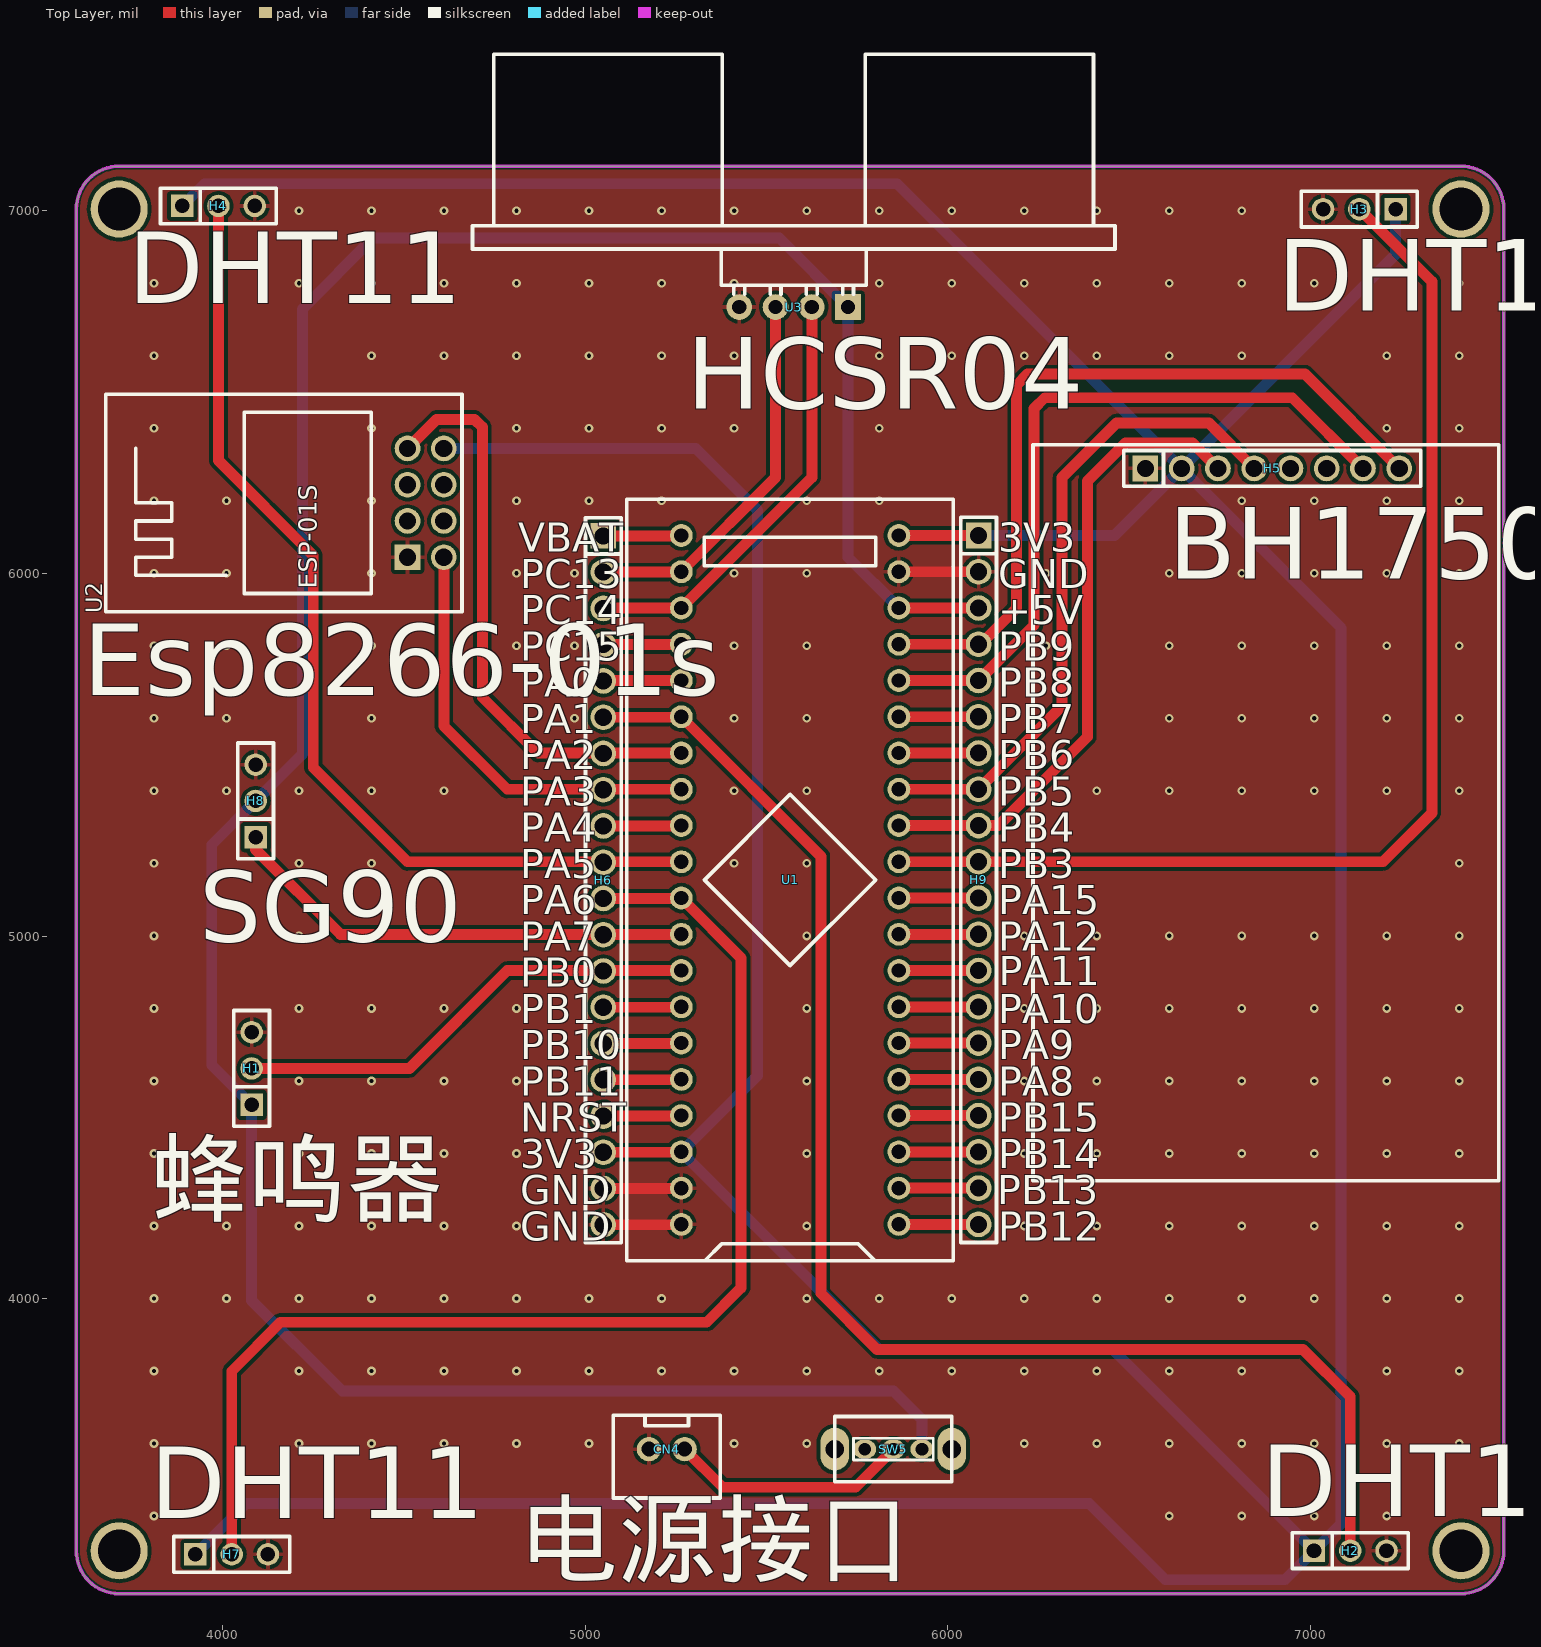
[diagram p0: Top Layer view]
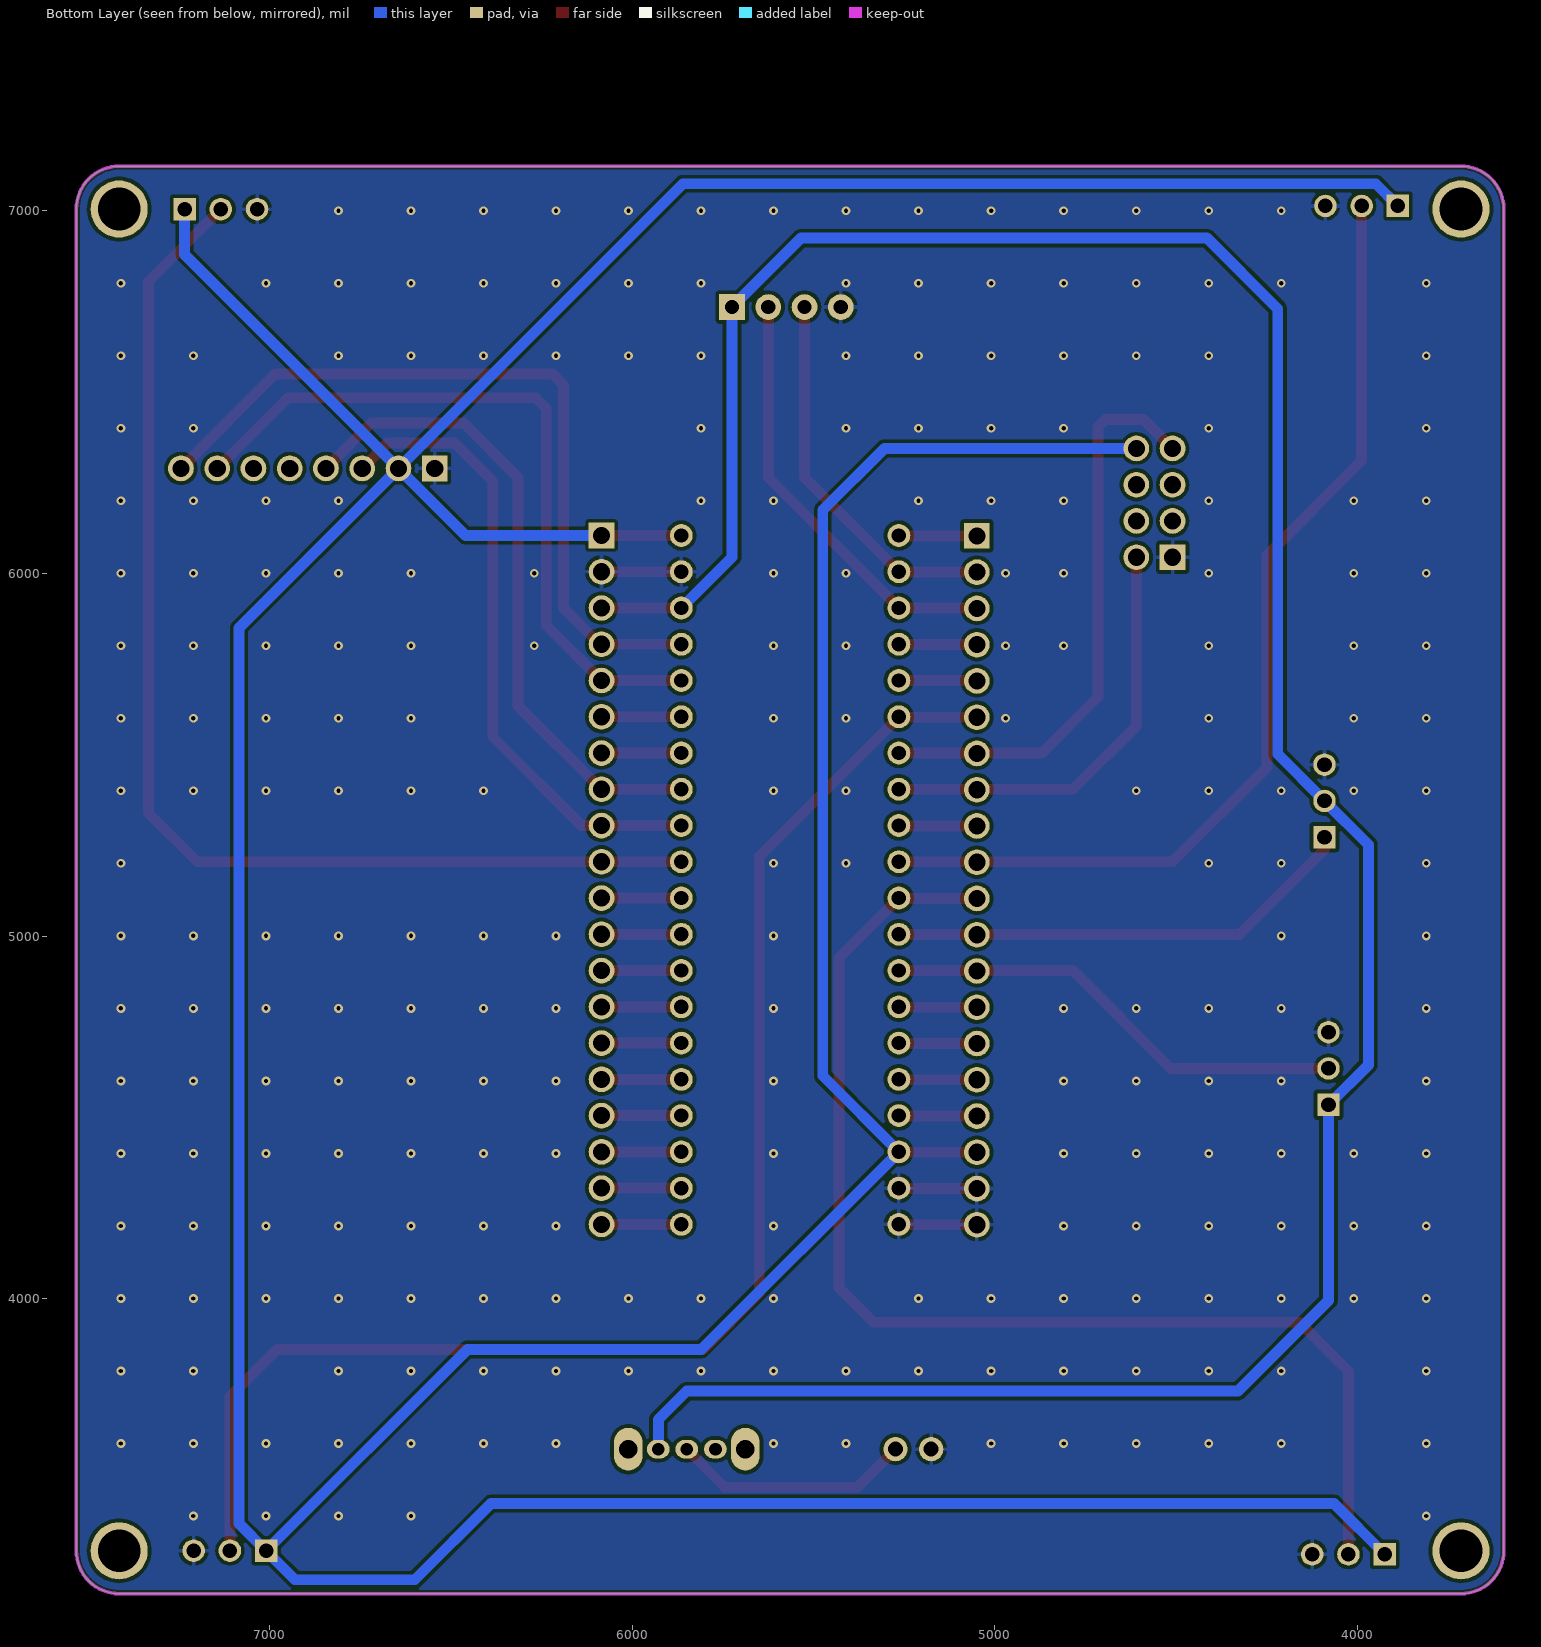
[diagram p1: Bottom Layer view, seen from below]
# Altium PCB MISC50977.pcbdoc
Units mil, origin at the board's own origin, x right, y up, seen from the top; angles counter-clockwise.
Board outline 3937.01 x 3937.01 mil, 2 copper layers (Top Layer, Bottom Layer), stack 62.206 mil thick; 14 components, 40 nets, 129 pads, 241 vias.

## Layer stack, top to bottom
Top Solder Mask Layer: solder mask 0.394, Dk 3.3
Top Layer: signal copper 1.379
Dielectric1: surface 59.449, FR4, Dk 4.5
Bottom Layer: signal copper 1.378
Bottom Solder Mask Layer: solder mask 0.394, Dk 3.3

## Board outline
3714.61,7123.5 ccw(c3714.61,7005.39) 3596.5,7005.39 3596.5,3304.61 ccw(c3714.61,3304.61) 3714.61,3186.5 7415.39,3186.5 ccw(c7415.39,3304.61) 7533.5,3304.61 7533.5,7005.39 ccw(c7415.39,7005.39) 7415.39,7123.5 3714.61,7123.5

## Design rules (kind name [scope] priority, off if disabled: settings)
BoardOutlineClearance copperThickness2oz_1 [All] p2 off: genericclearance=7.99 ignorepadtopadclearanceinfootprint=FALSE except(0: Arc-SplitContinuation Track-SplitContinuation SMDPad-SplitContinuation THPad-SplitContinuation Via-SplitContinuation Fill-SplitContinuation Region-SplitContinuation Poly-SplitContinuation Text-SplitContinuation Hole-SplitContinuation; 5.98: Arc-CutoutEdge SMDPad-CutoutEdge THPad-CutoutEdge Via-CutoutEdge Fill-CutoutEdge Region-CutoutEdge Text-CutoutEdge; 6.93: Hole-OutlineEdge Hole-CutoutEdge; 10: Poly-OutlineEdge Poly-CutoutEdge; 11.81: Arc-OutlineEdge Track-OutlineEdge SMDPad-OutlineEdge THPad-OutlineEdge Via-OutlineEdge Fill-OutlineEdge Region-OutlineEdge Text-OutlineEdge Track-CutoutEdge)
BoardOutlineClearance copperThickness1oz_1 [All] p4: genericclearance=4.02 ignorepadtopadclearanceinfootprint=FALSE except(0: Arc-SplitContinuation Track-SplitContinuation SMDPad-SplitContinuation THPad-SplitContinuation Via-SplitContinuation Fill-SplitContinuation Region-SplitContinuation Poly-SplitContinuation Text-SplitContinuation Hole-SplitContinuation; 6: SMDPad-CutoutEdge THPad-CutoutEdge Via-CutoutEdge Fill-CutoutEdge Region-CutoutEdge Text-CutoutEdge; 6.93: Hole-OutlineEdge Hole-CutoutEdge; 10: Poly-OutlineEdge Poly-CutoutEdge; 11.8: Arc-OutlineEdge Track-OutlineEdge SMDPad-OutlineEdge THPad-OutlineEdge Via-OutlineEdge Fill-OutlineEdge Region-OutlineEdge Text-OutlineEdge; 11.81: Arc-CutoutEdge Track-CutoutEdge)
Clearance copperThickness2oz [All] p1 off: gap=7.99 ignorepadtopadclearanceinfootprint=FALSE except(5.98: SMDPad-Track SMDPad-SMDPad THPad-Track SMDPad-THPad THPad-THPad Track-Via SMDPad-Via THPad-Via Via-Via Fill-Track Region-Track Fill-SMDPad Region-SMDPad Fill-THPad Region-THPad Fill-Via Region-Via Fill-Fill Fill-Region Region-Region Arc-Track Arc-SMDPad Arc-THPad Arc-Via Fill-Arc Region-Arc Arc-Arc Text-Track SMDPad-Text Text-THPad Text-Via Fill-Text Region-Text Arc-Text Text-Text; 6.93: Hole-Track Hole-SMDPad Hole-THPad Hole-Via Fill-Hole Region-Hole Hole-Arc Hole-Text; 10: Poly-Track Poly-SMDPad Poly-THPad Poly-Via Poly-Fill Poly-Region Poly-Poly Poly-Arc Poly-Text Poly-Hole)
Clearance copperThickness1oz [All] p3: gap=4.02 ignorepadtopadclearanceinfootprint=FALSE except(5.98: SMDPad-Track SMDPad-SMDPad THPad-Track SMDPad-THPad THPad-THPad Track-Via SMDPad-Via THPad-Via Via-Via Fill-Track Region-Track Fill-SMDPad Region-SMDPad Fill-THPad Region-THPad Fill-Via Region-Via Fill-Fill Fill-Region Region-Region; 6: Arc-Track Arc-SMDPad Arc-THPad Arc-Via Fill-Arc Region-Arc Arc-Arc Text-Track SMDPad-Text Text-THPad Text-Via Fill-Text Region-Text Arc-Text Text-Text; 6.93: Hole-Track Hole-SMDPad Hole-THPad Hole-Via Fill-Hole Region-Hole Hole-Arc Hole-Text; 10: Poly-Track Poly-SMDPad Poly-THPad Poly-Via Poly-Fill Poly-Region Poly-Poly Poly-Arc Poly-Text Poly-Hole)
DiffPairsRouting differentialPair [All] p1: maxlimit=6 minlimit=6 mostfreqgap=6 toplayer_minwidth=5 toplayer_prefwidth=10 toplayer_maxwidth=100 toplayer_mingap=6 toplayer_prefgap=6 toplayer_maxgap=6 bottomlayer_minwidth=5 bottomlayer_prefwidth=10 bottomlayer_maxwidth=100 bottomlayer_mingap=6 bottomlayer_prefgap=6 bottomlayer_maxgap=6 maxuncoupledlength=10
HoleToHoleClearance otherClearance [All] p1: gap=11.81 allowstackedmicrovias=TRUE
Length netLength [All] p1: minlimit=0 maxlimit=0
MatchedLengths netLengthTolerance [All] p1: tolerance=1000
PasteMaskExpansion pasteMaskExpansion [All] p1: expansion=0
PlaneConnect innerPlane [All] p1: planeconnectstyle=Relief reliefexpansion=20 reliefentries=4 reliefconductorwidth=10 reliefairgap=10
PolygonConnect copperRegion [All] p1: connectstyle=Relief reliefconductorwidth=10 reliefentries=4 polygonreliefangle="90 Angle" airgapwidth=10 via.connectstyle=Relief via.reliefconductorwidth=10 via.reliefentries=4 via.polygonreliefangle="90 Angle" via.airgapwidth=10
RoutingVias viaSize [All] p1: holewidth=12.01 width=24.02 viastyle="Through Hole" minholewidth=11.81 minwidth=19.68 maxholewidth=248.03 maxwidth=393.7
SolderMaskExpansion solderMaskExpansion [IsVia] p1: expansion=-1000 istentingtop=TRUE
SolderMaskExpansion solderMaskExpansion [All] p2: expansion=2 istentingtop=FALSE
Width copperThickness2oz_2 [All] p1 off: maxlimit=100 minlimit=8 preferedwidth=10
Width copperThickness1oz_2 [All] p2: maxlimit=100 minlimit=5 preferedwidth=10

## Components (designator, comment, footprint, x,y, rotation, side; value= is the part's Value field where it differs from the comment)
CN4 "XH2.54*2P_直插" CONN-TH_2P-P2.50-XH2.54-2P 5225,3585 r0 top
H1 "" HDR-TH_3P-P2.54-V-F 4080,4635 r90 top
H2 "" HDR-TH_3P-P2.54-V-F 7110,3305 r0 top
H3 "" HDR-TH_3P-P2.54-V-F 7135,7005 r180 top
H4 "" HDR-TH_3P-P2.54-V-F 3988.48,7013.84 r0 top
H5 "" HDR-TH_8P-P2.54-V-F-1 6895,6290 r0 top
H6 "" HDR-TH_20P-P2.54-V-M-1 5049.9,5153.84 r270 top
H7 "" HDR-TH_3P-P2.54-V-F 4025,3295 r0 top
H8 "" HDR-TH_3P-P2.54-V-F 4091.04,5372.91 r90 top
H9 "" HDR-TH_20P-P2.54-V-M-1 6085,5155 r270 top
SW5 "" 拨动开关 5855,3585 r180 top
U1 "STM32F103C8T6-Card" CONN-TH_L53.3-W22.9_STM32F103C8T6-CARD 5565,5155 r90 top
U2 "ESP-01S" WIFIM-TH_ESP-01S 4560,6195 r90 top
U3 "HC-SR04" TH_HC-SR04V 5575,6735 r180 top

## Footprints (in the part's own frame and the unit in brackets; to place one, negate y for a bottom-side part, rotate by r counter-clockwise, add the part's x,y. Pads: shape width x height; smd on the part's side, far side on the other; paste and mask are expansions set on the pad)
CONN-TH_2P-P2.50-XH2.54-2P [mm]
  round 1.7 hole 1.05 paste+0 mask+0.05: 1(1.25,0) 2(-1.25,0)
  silkscreen extent -3.75,-3.42 3.75,2.37
CONN-TH_L53.3-W22.9_STM32F103C8T6-CARD [mm]
  round 1.6 hole 1: 1(-24.13,-7.62) 2(-21.59,-7.62) 3(-19.05,-7.62) 4(-16.51,-7.62) 5(-13.97,-7.62) 6(-11.43,-7.62) 7(-8.89,-7.62) 8(-6.35,-7.62) 9(-3.81,-7.62) 10(-1.27,-7.62) 11(1.27,-7.62) 12(3.81,-7.62) 13(6.35,-7.62) 14(8.89,-7.62) 15(11.43,-7.62) 16(13.97,-7.62) 17(16.51,-7.62) 18(19.05,-7.62) 19(21.59,-7.62) 20(24.13,-7.62) 21(24.13,7.62) 22(21.59,7.62) 23(19.05,7.62) 24(16.51,7.62) 25(13.97,7.62) 26(11.43,7.62) 27(8.89,7.62) 28(6.35,7.62) 29(3.81,7.62) 30(1.27,7.62) 31(-1.27,7.62) 32(-3.81,7.62) 33(-6.35,7.62) 34(-8.89,7.62) 35(-11.43,7.62) 36(-13.97,7.62) 37(-16.51,7.62) 38(-19.05,7.62) 39(-21.59,7.62) 40(-24.13,7.62)
  silkscreen extent -26.67,-11.43 26.67,11.43
HDR-TH_3P-P2.54-V-F [mil]
  rect 62x62 hole 40.16: 1(-100,0)
  round 62 hole 40.16: 2(0,0) 3(100,0)
  silkscreen extent -160,-49 160,49
HDR-TH_8P-P2.54-V-F-1 [mm]
  rect 1.8x1.8 hole 1.2: 1(-8.89,0)
  round 1.8 hole 1.2: 2(-6.35,0) 3(-3.81,0) 4(-1.27,0) 5(1.27,0) 6(3.81,0) 7(6.35,0) 8(8.89,0)
  silkscreen extent -10.41,-1.25 10.41,1.25
HDR-TH_20P-P2.54-V-M-1 [mm]
  rect 1.8x1.8 hole 1.2: 1(-24.13,0)
  round 1.8 hole 1.2: 2(-21.59,0) 3(-19.05,0) 4(-16.51,0) 5(-13.97,0) 6(-11.43,0) 7(-8.89,0) 8(-6.35,0) 9(-3.81,0) 10(-1.27,0) 11(1.27,0) 12(3.81,0) 13(6.35,0) 14(8.89,0) 15(11.43,0) 16(13.97,0) 17(16.51,0) 18(19.05,0) 19(21.59,0) 20(24.13,0)
  silkscreen extent -25.4,-1.25 25.4,1.25
TH_HC-SR04V [mm]
  rect 1.8x1.8 hole 1.001: 1(-3.81,0)
  round 1.8 hole 1.001: 2(-1.27,0) 3(1.27,0) 4(3.81,0)
  silkscreen extent -22.5,-17.7 22.5,-0.89
WIFIM-TH_ESP-01S [mm]
  rect 1.8x1.8 hole 1.2: 1(-3.81,1.27)
  round 1.8 hole 1.2: 2(-1.27,1.27) 3(1.27,1.27) 4(3.81,1.27) 5(3.81,-1.27) 6(1.27,-1.27) 7(-1.27,-1.27) 8(-3.81,-1.27)
  silkscreen extent -7.62,-2.54 7.62,22.4
拨动开关 [mil]
  oval 63x51.2 hole 35.4 paste+0 mask+2: 1(-73.4,0) 2(5,0) 3(84,0)
  oval 78.7x118.1 hole 51.2 paste+0 mask+2: 4(166.7,0) 5(-156.1,0)
  silkscreen extent -156,-90 167,90

## Free pads (board coordinates)
  round 157.48 hole 118.11: 1(3714.61,7005.39) 1(3714.61,3304.61) 1(7415.39,7005.39) 1(7415.39,3304.61)

## Via types
v1: diameter 24.02, hole 12, Top Layer to Bottom Layer, 241 vias

## Nets (pads, with @x,y where several pads share a name; then routed paths per layer and width w, separated by ;. In a path a pad name is that pad's centre, name@x,y a point inside that pad or via, vN(x,y) a via of type N, cw(c..) or ccw(c..) an arc to the next point about the centre after c; other vN are vias at no path point)
$1N9: CN4.1 SW5.2 | length 662.8
  Top Layer w30: CN4.1 5379.22,3480 5745,3480 SW5.2
+5V: H1.1 H8.2 H9.3 SW5.1 U1.18 U3.1 | length 7722.6
  Top Layer w30: U1.18 H9.3
  Bottom Layer w30: U1.18 5725,6045 U3.1 5535,6925 4415,6925 4220,6730 4220,5501.87 H8.2 3970,5251.87 3970,4645 H1.1 4080,3995 4330,3745 5850,3745 5928.4,3666.6 SW5.1
GND: CN4.2 H1.3 H2.3 H3.3 H4.3 H5.1 H6.19 H6.20 H7.3 H8.3 H9.2 U1.19 U1.39 U1.40 U2.1 U3.4 | length 651.2
  Top Layer w30: H6.20 5263.83,4203.84 U1.40 ; H6.19 5263.83,4303.84 U1.39 ; U1.19 H9.2
  other v1: 3810.6,3400.6 6610.6,3400.6 6810.6,3400.6 7010.6,3400.6 7210.6,3400.6 3810.6,3600.6 4210.6,3600.6 4410.6,3600.6 4610.6,3600.6 4810.6,3600.6 5010.6,3600.6 5410.6,3600.6 5610.6,3600.6 6210.6,3600.6 6410.6,3600.6 6610.6,3600.6 6810.6,3600.6 7010.6,3600.6 7210.6,3600.6 7410.6,3600.6 3810.6,3800.6 4210.6,3800.6 4410.6,3800.6 4610.6,3800.6 4810.6,3800.6 5010.6,3800.6 5210.6,3800.6 5410.6,3800.6 5610.6,3800.6 5810.6,3800.6 6010.6,3800.6 6210.6,3800.6 6410.6,3800.6 6610.6,3800.6 6810.6,3800.6 7210.6,3800.6 7410.6,3800.6 3810.6,4000.6 4010.6,4000.6 4210.6,4000.6 4410.6,4000.6 4610.6,4000.6 4810.6,4000.6 5010.6,4000.6 5210.6,4000.6 5610.6,4000.6 5810.6,4000.6 6010.6,4000.6 6210.6,4000.6 6410.6,4000.6 6610.6,4000.6 6810.6,4000.6 7010.6,4000.6 7210.6,4000.6 7410.6,4000.6 3810.6,4200.6 4010.6,4200.6 4210.6,4200.6 4410.6,4200.6 4610.6,4200.6 4810.6,4200.6 5610.6,4200.6 6210.6,4200.6 6410.6,4200.6 6610.6,4200.6 6810.6,4200.6 7010.6,4200.6 7210.6,4200.6 7410.6,4200.6 3810.6,4400.6 4010.6,4400.6 4210.6,4400.6 4410.6,4400.6 4610.6,4400.6 4810.6,4400.6 5610.6,4400.6 6210.6,4400.6 6410.6,4400.6 6610.6,4400.6 6810.6,4400.6 7010.6,4400.6 7210.6,4400.6 7410.6,4400.6 3810.6,4600.6 4210.6,4600.6 4410.6,4600.6 4610.6,4600.6 4810.6,4600.6 5610.6,4600.6 6210.6,4600.6 6410.6,4600.6 6610.6,4600.6 6810.6,4600.6 7010.6,4600.6 7210.6,4600.6 7410.6,4600.6 3810.6,4800.6 4210.6,4800.6 4410.6,4800.6 4610.6,4800.6 4810.6,4800.6 5610.6,4800.6 6210.6,4800.6 6410.6,4800.6 6610.6,4800.6 6810.6,4800.6 7010.6,4800.6 7210.6,4800.6 7410.6,4800.6 3810.6,5000.6 4210.6,5000.6 5610.6,5000.6 6210.6,5000.6 6410.6,5000.6 6610.6,5000.6 6810.6,5000.6 7010.6,5000.6 7210.6,5000.6 7410.6,5000.6 3810.6,5200.6 4210.6,5200.6 4410.6,5200.6 5410.6,5200.6 5610.6,5200.6 7410.6,5200.6 3810.6,5400.6 4010.6,5400.6 4210.6,5400.6 4410.6,5400.6 4610.6,5400.6 5410.6,5400.6 5610.6,5400.6 6410.6,5400.6 6610.6,5400.6 6810.6,5400.6 7010.6,5400.6 7210.6,5400.6 7410.6,5400.6 3810.6,5600.6 4010.6,5600.6 4410.6,5600.6 4970.6,5600.6 5410.6,5600.6 5610.6,5600.6 6610.6,5600.6 6810.6,5600.6 7010.6,5600.6 7210.6,5600.6 7410.6,5600.6 3810.6,5800.6 4010.6,5800.6 4410.6,5800.6 4810.6,5800.6 4970.6,5800.6 5410.6,5800.6 5610.6,5800.6 6270.6,5800.6 6610.6,5800.6 6810.6,5800.6 7010.6,5800.6 7210.6,5800.6 7410.6,5800.6 3810.6,6000.6 4010.6,6000.6 4410.6,6000.6 4810.6,6000.6 4970.6,6000.6 5410.6,6000.6 5610.6,6000.6 6270.6,6000.6 6610.6,6000.6 6810.6,6000.6 7010.6,6000.6 7210.6,6000.6 7410.6,6000.6 3810.6,6200.6 4010.6,6200.6 4410.6,6200.6 4810.6,6200.6 5010.6,6200.6 5210.6,6200.6 5610.6,6200.6 5810.6,6200.6 6810.6,6200.6 7010.6,6200.6 7210.6,6200.6 7410.6,6200.6 3810.6,6400.6 4410.6,6400.6 4810.6,6400.6 5010.6,6400.6 5210.6,6400.6 5410.6,6400.6 5810.6,6400.6 7210.6,6400.6 7410.6,6400.6 3810.6,6600.6 4410.6,6600.6 4610.6,6600.6 4810.6,6600.6 5010.6,6600.6 5210.6,6600.6 5410.6,6600.6 5810.6,6600.6 6010.6,6600.6 6210.6,6600.6 6410.6,6600.6 6610.6,6600.6 6810.6,6600.6 7210.6,6600.6 7410.6,6600.6 3810.6,6800.6 4210.6,6800.6 4410.6,6800.6 4610.6,6800.6 4810.6,6800.6 5010.6,6800.6 5210.6,6800.6 5410.6,6800.6 5810.6,6800.6 6010.6,6800.6 6210.6,6800.6 6410.6,6800.6 6610.6,6800.6 6810.6,6800.6 7010.6,6800.6 7410.6,6800.6 4210.6,7000.6 4410.6,7000.6 4610.6,7000.6 4810.6,7000.6 5010.6,7000.6 5210.6,7000.6 5410.6,7000.6 5610.6,7000.6 5810.6,7000.6 6010.6,7000.6 6210.6,7000.6 6410.6,7000.6 6610.6,7000.6 6810.6,7000.6
NRST: H6.17 U1.37 | length 215.6
  Top Layer w30: H6.17 5263.83,4503.84 U1.37
PA0: H6.5 U1.25 | length 215.6
  Top Layer w30: H6.5 5051.06,5705 U1.25
PA1: H2.2 H6.6 U1.26 | length 3968.1
  Top Layer w30: H6.6 5263.83,5603.84 U1.26 5650,5220 5650,4015 5805,3860 6980,3860 7110,3730 H2.2
PA2: H6.7 U1.27 U2.4 | length 1605.6
  Top Layer w30: U2.4 4590,6425 4695,6425 4716.21,6403.79 4716.21,5658.79 4870,5505 U1.27
PA3: H6.8 U1.28 U2.8 | length 1192.5
  Top Layer w30: U2.8 4610,5580 4785,5405 U1.28
PA4: H6.9 U1.29 | length 215.6
  Top Layer w30: H6.9 5263.83,5303.84 U1.29
PA5: H4.2 H6.10 U1.30 | length 2779.9
  Top Layer w30: H4.2 3988.48,6311.52 4250,6050 4250,5465 4510,5205 U1.30
PA6: H6.11 H7.2 U1.31 | length 3364.2
  Top Layer w30: H7.2 4025,3800 4160,3935 5335,3935 5430,4030 5430,4940 U1.31 5263.83,5103.84 H6.11
PA7: H6.12 H8.1 U1.32 | length 1304.8
  Top Layer w30: H8.1 4091.04,5238.96 4325,5005 U1.32
PA8: H9.16 U1.5 | length 220
  Top Layer w30: U1.5 H9.16
PA9: H9.15 U1.6 | length 220
  Top Layer w30: U1.6 H9.15
PA10: H9.14 U1.7 | length 220
  Top Layer w30: U1.7 H9.14
PA11: H9.13 U1.8 | length 220
  Top Layer w30: U1.8 H9.13
PA12: H9.12 U1.9 | length 220
  Top Layer w30: U1.9 H9.12
PA15: H9.11 U1.10 | length 220
  Top Layer w30: U1.10 H9.11
PB0: H1.2 H6.13 U1.33 | length 1296.8
  Top Layer w30: H1.2 4515,4635 4785,4905 U1.33
PB1: H6.14 U1.34 | length 215.6
  Top Layer w30: H6.14 5263.83,4803.84 U1.34
PB3: H3.2 H9.10 U1.11 | length 3273.8
  Top Layer w30: U1.11 H9.10 7200,5205 7335,5340 7335,6805 H3.2
PB4: H5.3 H9.9 U1.12 | length 1759
  Top Layer w30: U1.12 H9.9 6140,5305 6385,5550 6385,6255 6490,6360 6675,6360 H5.3
PB5: H5.4 H9.8 U1.13 | length 1819.2
  Top Layer w30: U1.13 H9.8 6315,5635 6315,6265 6465,6415 6720,6415 H5.4
PB6: H5.5
PB7: H5.6
PB8: H5.7 H9.5 U1.16 | length 2033.8
  Top Layer w30: U1.16 H9.5 6237.6,5857.6 6237.6,6455 6267.6,6485 6950,6485 H5.7
PB9: H5.8 H9.4 U1.17 | length 2156.5
  Top Layer w30: U1.17 6090,5805 6190,5905 6190,6520 6220,6550 6985,6550 H5.8
PB10: H6.15 U1.35 | length 215.6
  Top Layer w30: H6.15 5263.83,4703.84 U1.35
PB11: H6.16 U1.36 | length 215.6
  Top Layer w30: H6.16 5263.83,4603.84 U1.36
PB12: H9.20 U1.1 | length 220
  Top Layer w30: U1.1 H9.20
PB13: H9.19 U1.2 | length 220
  Top Layer w30: U1.2 H9.19
PB14: H9.18 U1.3 | length 220
  Top Layer w30: U1.3 H9.18
PB15: H9.17 U1.4 | length 220
  Top Layer w30: U1.4 H9.17
PC13: H6.2 U1.22 U3.3 | length 1053.3
  Top Layer w30: H6.2 5263.83,6003.84 U1.22 5525,6265 U3.3
PC14: H6.3 U1.23 U3.2 | length 1194.7
  Top Layer w30: H6.3 5051.06,5905 U1.23 5625,6265 U3.2
PC15: H6.4 U1.24 | length 215.6
  Top Layer w30: H6.4 5263.83,5803.84 U1.24
SCL: H9.7 U1.14 | length 220
  Top Layer w30: U1.14 H9.7
SDA: H9.6 U1.15 | length 220
  Top Layer w30: U1.15 H9.6
VBAT: H6.1 U1.21 | length 215.6
  Top Layer w30: H6.1 5263.83,6103.84 U1.21
VCC: H2.1 H3.1 H4.1 H5.2 H6.18 H7.1 H9.1 U1.20 U1.38 U2.5 | length 16593.2
  Top Layer w30: H6.18 5263.83,4403.84 U1.38 ; U1.20 H9.1
  Bottom Layer w30: H4.1 3949.64,7075 5860,7075 6592.18,6342.82 cw(c6580.43,6325.43) 6597.82,6337.18 H5.2 ; H7.1 4065,3435 6390,3435 6600,3225 6930,3225 H2.1 ; U2.5 5305,6345 5475,6175 5475,4615 U1.38 5810,3860 6455,3860 H2.1 ; H9.1 6460,6105 6592.18,6237.18 ccw(c6580.43,6254.57) 6597.82,6242.82 H5.2 ; H3.1 7235,6880 H5.2 ; H5.2 7085,5850 7085,3380 H2.1
pads on no net: SW5.3 SW5.4 SW5.5 U2.2 U2.3 U2.6 U2.7

## Polygon pours and split planes (outlines as drawn)
GND on Bottom Layer (solid, remove dead copper, pour order 2): 3525,7245 3525,3080 7700,3080 7700,7245
GND on Top Layer (solid, remove dead copper, pour order 2): 3000,7415 3000,3000 7930,3000 7930,7415

## Keep-outs
Board Outline Layer:
  the board outline again, w10

## Silkscreen, mask and mechanical layers (free items; w line width, h text height)
Top Silkscreen Layer:
  lines w10: 6235,4325 6235,6355 7520,6355 7520,4325 6235,4325
  text "DHT11" at 3740,6745 h196.85
  text "DHT11" at 6910,6725 h196.85
  text "HCSR04" at 5280,6455 h196.85
  text "VBAT" at 4815.95,6060 h80
  text "3V3" at 6139.16,6060 h80
  text "BH1750" at 6610,5985 h196.85
  text "PC13" at 4820.95,5960 h80
  text "GND" at 6139.16,5960 h80
  text "PC14" at 4820.95,5860 h80
  text "+5V" at 6139.16,5860 h80
  text "PC15" at 4820.95,5760 h80
  text "PB9" at 6139.16,5760 h80
  text "Esp8266-01s" at 3615,5665 h196.85
  text "PA0" at 4820.95,5660 h80
  text "PB8" at 6139.16,5660 h80
  text "PA1" at 4820.95,5560 h80
  text "PB7" at 6139.16,5560 h80
  text "PA2" at 4820.95,5460 h80
  text "PB6" at 6139.16,5460 h80
  text "PA3" at 4820.95,5360 h80
  text "PB5" at 6139.16,5360 h80
  text "PA4" at 4820.95,5260 h80
  text "PB4" at 6139.16,5260 h80
  text "PA5" at 4820.95,5160 h80
  text "PB3" at 6139.16,5160 h80
  text "PA6" at 4820.95,5060 h80
  text "PA15" at 6139.16,5060 h80
  text "SG90" at 3935,4985 h196.85
  text "PA7" at 4820.95,4960 h80
  text "PA12" at 6139.16,4960 h80
  text "PA11" at 6140.95,4865 h80
  text "PB0" at 4820.95,4860 h80
  text "PB1" at 4820.95,4760 h80
  text "PA10" at 6139.16,4760 h80
  text "PB10" at 4820.95,4660 h80
  text "PA9" at 6139.16,4660 h80
  text "PB11" at 4820.95,4560 h80
  text "PA8" at 6139.16,4560 h80
  text "NRST" at 4820.95,4460 h80
  text "PB15" at 6139.16,4460 h80
  text "3V3" at 4820.95,4360 h80
  text "PB14" at 6139.16,4360 h80
  text "GND" at 4820.95,4260 h80
  text "PB13" at 6135.95,4260 h80
  text "蜂鸣器" at 3800,4235 h196.85
  text "GND" at 4820.95,4160 h80
  text "PB12" at 6139.16,4160 h80
  text "DHT11" at 6865,3400 h196.85
  text "DHT11" at 3800,3395 h196.85
  text "电源接口" at 4822.87,3241.57 h196.85